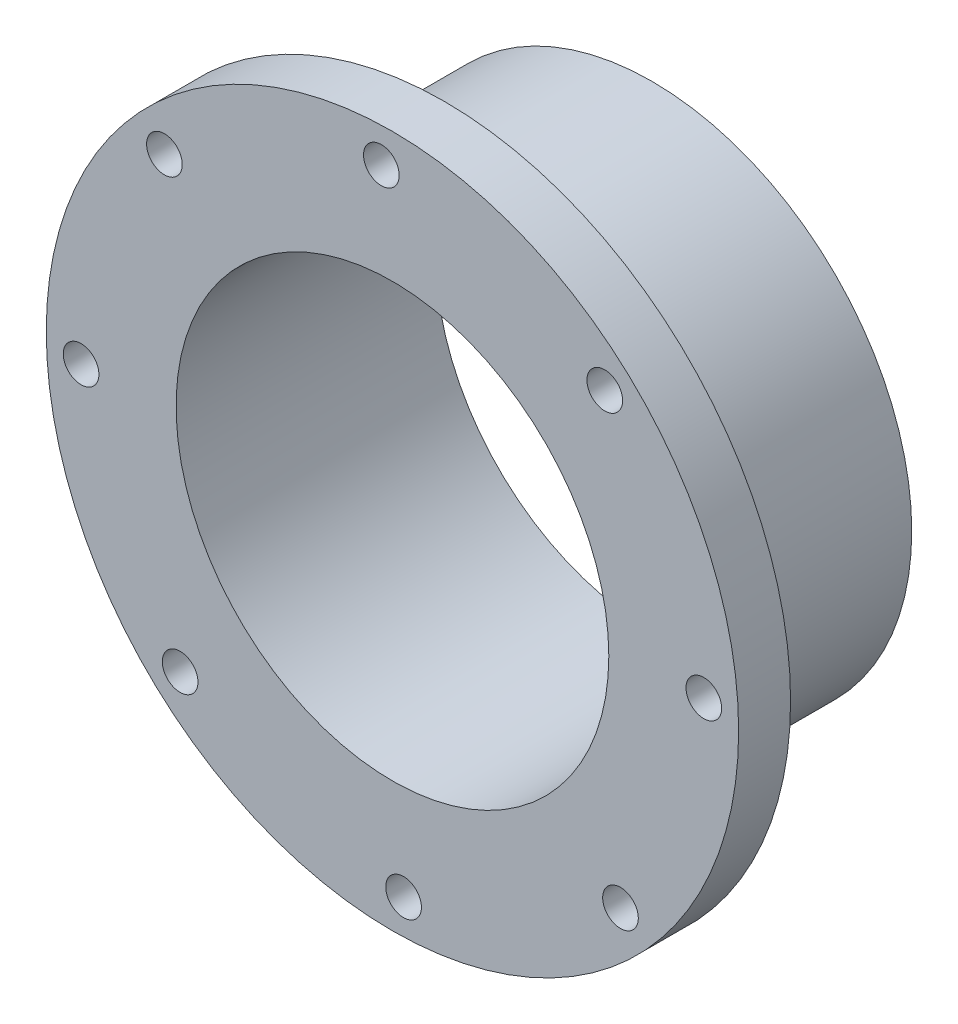
SolidWorks part; units mm, degrees
ref_plane "Front Plane" through (0, 0, 0) normal (0, 0, 1) x (1, 0, 0)
ref_plane "Top Plane" through (0, 0, 0) normal (0, 1, 0) x (1, 0, 0)
ref_plane "Right Plane" through (0, 0, 0) normal (1, 0, 0) x (0, 0, -1)
sketch "Sketch1" plane through (0, 0, 0) normal (0, 0, 1) x (1, 0, 0)
  circle A0 centre (0, 0) radius 12.5
  circle A1 centre (0, 0) radius 15
  dimension "D1" = 25
  dimension "D2" = 30
extrude "Boss-Extrude1" add sketch "Sketch1" along normal blind 5
sketch "Sketch2" plane through (0, 0, 5) normal (0, 0, 1) x (1, 0, 0)
  circle A0 centre (0, 0) radius 12.5
  circle A1 centre (0, 0) radius 15
extrude "Boss-Extrude2" add sketch "Sketch2" along normal blind 10
sketch "Sketch3" plane through (0, 0, 12) normal (0, 0, 1) x (1, 0, 0)
  circle A1 centre (0, 0) radius 20
  circle A2 centre (0, 0) radius 14.8858
extrude "Boss-Extrude5" add sketch "Sketch3" along normal up to surface (3 mm away) up to face at (15, 0, 15)
sketch "Sketch6" plane through (0, 0, 15) normal (0, 0, 1) x (1, 0, 0)
  circle A0 centre (0, 0) radius 18 construction
  circle A1 centre (17.9886, 0.6417) radius 1.03
  circle A7 centre (13.1736, -12.2661) radius 1.03
  circle A8 centre (0.6417, -17.9886) radius 1.03
  circle A9 centre (-12.2661, -13.1736) radius 1.03
  circle A10 centre (-17.9886, -0.6417) radius 1.03
  circle A11 centre (-13.1736, 12.2661) radius 1.03
  circle A12 centre (-0.6417, 17.9886) radius 1.03
  circle A13 centre (12.2661, 13.1736) radius 1.03
  point P17 (0, 0)
  point P22 (0, 0)
  dimension "D1" = 36
  dimension "D2" = 2.06
  dimension "D3" = 8
extrude "Cut-Extrude9" cut sketch "Sketch6" against normal blind 10
